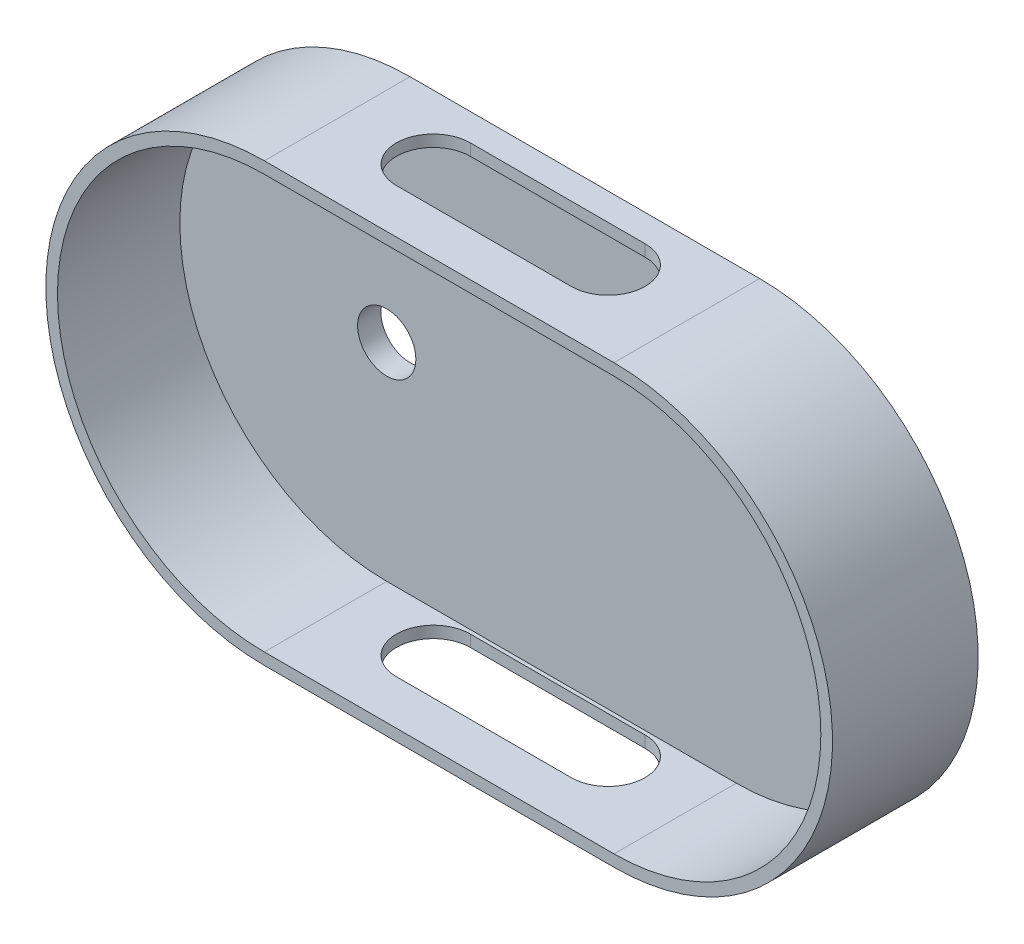
from build123d import *

# Parameters (mm, degrees)
SKETCH1_R           = 5
BOSS_EXTRUDE1_DEPTH = 25
CUT_EXTRUDE1_DEPTH  = 21
CUT_EXTRUDE2_DEPTH  = 21


with BuildPart() as part:
    # Sketch1 → Boss-Extrude1 (new body)
    with BuildSketch(Plane.XY):
        with BuildLine():
            Line((0, 37.5), (60, 37.5))
            ThreePointArc((60, 37.5), (97.5, 0), (60, -37.5))
            Line((60, -37.5), (0, -37.5))
            ThreePointArc((0, -37.5), (-37.5, 0), (0, 37.5))
        make_face()
        Circle(SKETCH1_R, mode=Mode.SUBTRACT)
    extrude(amount=BOSS_EXTRUDE1_DEPTH)

    # Sketch2 → Cut-Extrude1 (cut)
    with BuildSketch(Plane.XY.offset(25)):
        with BuildLine():
            Line((60, 35.5), (0, 35.5))
            ThreePointArc((0, 35.5), (-35.5, 0), (0, -35.5))
            Line((0, -35.5), (60, -35.5))
            ThreePointArc((60, -35.5), (95.5, 0), (60, 35.5))
        make_face()
    extrude(amount=-CUT_EXTRUDE1_DEPTH, mode=Mode.SUBTRACT)

    # Sketch4 → Cut-Extrude2 (cut)
    with BuildSketch(Plane.XZ.offset(37.5)):
        with BuildLine():
            Line((15, 17.341846587), (45, 17.341846587))
            ThreePointArc((45, 17.341846587), (51.341846587, 11), (45, 4.658153413))
            Line((45, 4.658153413), (15, 4.658153413))
            ThreePointArc((15, 4.658153413), (8.658153413, 11), (15, 17.341846587))
        make_face()
    cut_extrude2 = extrude(amount=-CUT_EXTRUDE2_DEPTH, mode=Mode.SUBTRACT)

    # Mirror2: Cut-Extrude2 across plane
    add(cut_extrude2.mirror(Plane.ZX), mode=Mode.SUBTRACT)


solid = part.part
